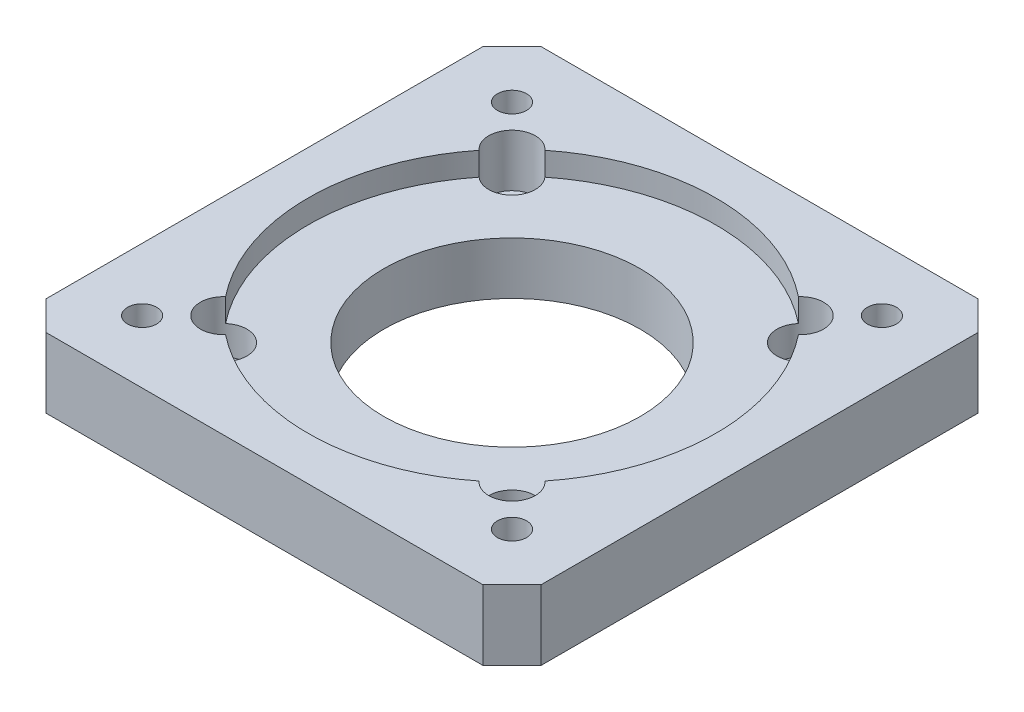
SolidWorks part; units mm, degrees
material "6061Al"
ref_plane "前视基准面" through (0, 0, 0) normal (0, 0, 1) x (1, 0, 0)
ref_plane "上视基准面" through (0, 0, 0) normal (0, 1, 0) x (1, 0, 0)
ref_plane "右视基准面" through (0, 0, 0) normal (1, 0, 0) x (0, 0, -1)
sketch "草图1" plane through (0, 0, 0) normal (0, 1, 0) x (1, 0, 0)
  line L1 (-42.5, -42.5) -> (42.5, -42.5)
  line L2 (-42.5, -42.5) -> (-42.5, 42.5)
  line L3 (-42.5, 42.5) -> (42.5, 42.5)
  line L4 (42.5, -42.5) -> (42.5, 42.5)
  line L5 (-42.5, -42.5) -> (42.5, 42.5) construction
  line L6 (-42.5, 42.5) -> (42.5, -42.5) construction
  point P0 (0, 0)
  dimension "D1" = 85
extrude "凸台-拉伸1" add sketch "草图1" along normal mid plane 12
sketch "草图2" plane through (0, -6, 0) normal (0, -1, 0) x (1, 0, 0)
  circle A0 centre (0, 0) radius 25
  dimension "D1" = 50
extrude "凸台-拉伸2" add sketch "草图2" along normal mid plane 2
sketch "草图3" plane through (0, -7, 0) normal (0, -1, 0) x (1, 0, 0)
  circle A0 centre (0, 0) radius 22
  circle A1 centre (0, 0) radius 25
  circle A2 centre (0, 0) radius 25 construction
  dimension "D1" = 0
  dimension "D2" = 3
extrude "切除-拉伸1" cut sketch "草图3" against normal through all
sketch "草图4" plane through (0, 6, 0) normal (0, 1, 0) x (1, 0, 0)
  circle A0 centre (0, 0) radius 35
  dimension "D1" = 70
extrude "切除-拉伸2" cut sketch "草图4" against normal blind 4
hole_wizard "M6 螺纹孔1" positions "草图5" profile "草图6" tap size "M6" standard "ISO" end condition through all
sketch "草图5" plane through (0, 6, 0) normal (0, 1, 0) x (1, 0, 0)
  line L1 (31.75, -31.75) -> (-31.75, -31.75)
  line L2 (31.75, -31.75) -> (31.75, 31.75)
  line L3 (31.75, 31.75) -> (-31.75, 31.75)
  line L4 (-31.75, -31.75) -> (-31.75, 31.75)
  line L5 (31.75, -31.75) -> (-31.75, 31.75) construction
  line L6 (31.75, 31.75) -> (-31.75, -31.75) construction
  point P0 (-31.75, 31.75)
  point P3 (0, 0)
  point P7 (31.75, -31.75)
  point P8 (31.75, 31.75)
  point P9 (-31.75, -31.75)
  dimension "D1" = 63.5
sketch "草图6" plane through (-31.75, 6, -31.75) normal (1, 0, 0) x (0, 0, 1)
  line L0 (0, 0) -> (0, 13)
  line L1 (0, 13) -> (2.5, 13)
  line L2 (2.5, 13) -> (2.5, 0)
  line L5 (2.5, 0) -> (0, 0)
  line L11 (0, -6.35) -> (0, 107.95) construction
  dimension "通孔螺纹孔钻头直径" = 5
  dimension "通孔螺纹孔钻头深度" = 13
cosmetic thread "孔螺蚊线1" parameters "D2"=6
cosmetic thread "孔螺蚊线2" parameters "D2"=6
cosmetic thread "孔螺蚊线3" parameters "D2"=6
cosmetic thread "孔螺蚊线4" parameters "D2"=6
chamfer "倒角1" distance 5 angle 45 4 edges at (-42.5, 0, 42.5) (42.5, 0, 42.5) (42.5, 0, -42.5) (-42.5, 0, -42.5)
hole_wizard "PZ-000000C 铺砖车" positions "草图7" profile "草图8" counterbore size "M4" standard "ISO" end condition through all
sketch "草图7" plane through (0, 6, 0) normal (0, 1, 0) x (1, 0, 0)
  point P0 (-24.7487, 24.7487)
  point P3 (24.7487, 24.7487)
  point P6 (24.7487, -24.7487)
  point P9 (-24.7487, -24.7487)
sketch "草图8" plane through (-24.7487, 6, -24.7487) normal (1, 0, 0) x (0, 0, 1)
  line L0 (0, 0) -> (0, 13)
  line L1 (0, 13) -> (2.25, 13)
  line L3 (2.25, 13) -> (2.25, 9)
  line L4 (2.25, 9) -> (4, 9)
  line L5 (4, 9) -> (4, 0)
  line L7 (4, 0) -> (0, 0)
  line L11 (0, -6.35) -> (0, 107.95) construction
  dimension "通孔孔直径" = 4.5
  dimension "通孔孔深度" = 13
  dimension "柱形沉头孔直径" = 8
  dimension "柱形沉头孔深度" = 9
